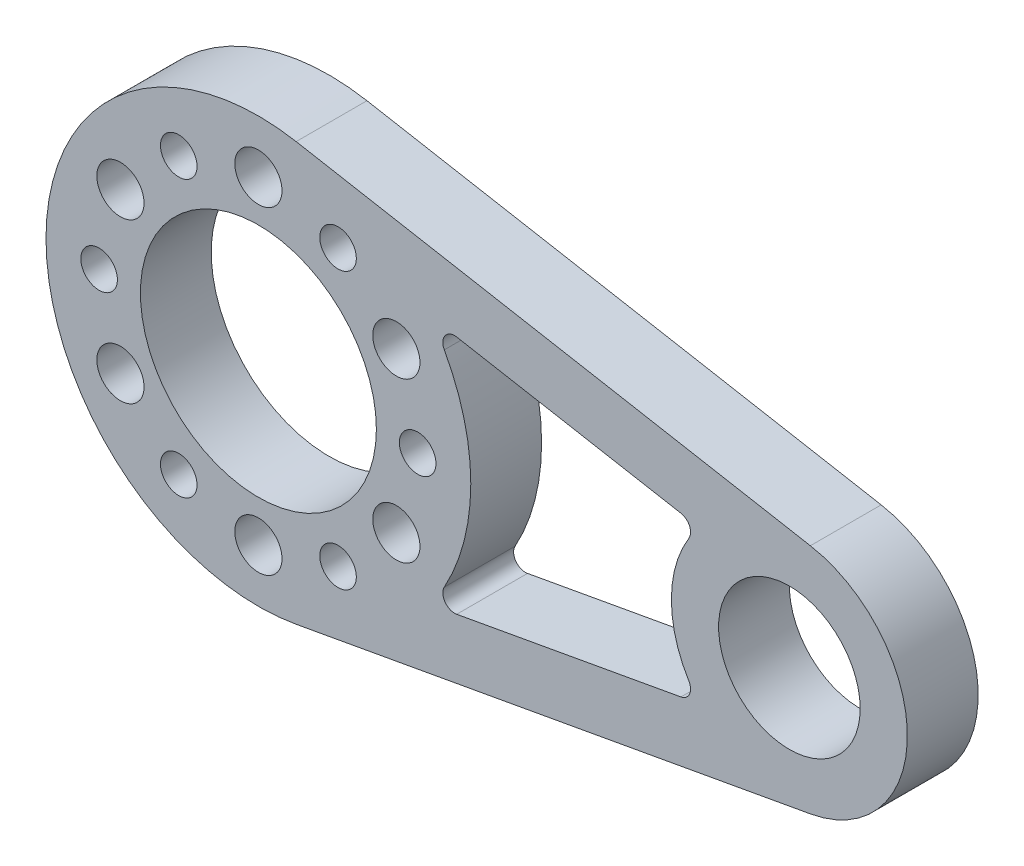
from build123d import *

# Parameters (mm, degrees)
SKETCH_1_R          = 2
SKETCH_1_R_2        = 1.55
SKETCH_1_R_3        = 10
SKETCH_1_R_4        = 6
EXTRUDE_1_DEPTH     = 6
CUT_EXTRUDE_1_DEPTH = 59.180752831
FILLET_1_R          = 1


with BuildPart() as part:
    # 草图1 → 凸台-拉伸1 (new body)
    with BuildSketch(Plane.XY):
        with BuildLine():
            Line((46.777777778, 9.840706589), (3.2, 17.71327186))
            ThreePointArc((3.2, 17.71327186), (-18, 0), (3.2, -17.71327186))
            Line((3.2, -17.71327186), (46.777777778, -9.840706589))
            ThreePointArc((46.777777778, -9.840706589), (55, 0), (46.777777778, 9.840706589))
        make_face()
        with Locations((0, 13.5)):
            Circle(SKETCH_1_R, mode=Mode.SUBTRACT)
        with Locations((6.75, 11.691342951)):
            Circle(SKETCH_1_R_2, mode=Mode.SUBTRACT)
        with Locations((0, -13.5)):
            Circle(SKETCH_1_R, mode=Mode.SUBTRACT)
        with Locations((-6.75, -11.691342951)):
            Circle(SKETCH_1_R_2, mode=Mode.SUBTRACT)
        with Locations((6.75, -11.691342951)):
            Circle(SKETCH_1_R_2, mode=Mode.SUBTRACT)
        with Locations((-11.691342951, -6.75)):
            Circle(SKETCH_1_R, mode=Mode.SUBTRACT)
        with Locations((11.691342951, -6.75)):
            Circle(SKETCH_1_R, mode=Mode.SUBTRACT)
        with Locations((-13.5, 0)):
            Circle(SKETCH_1_R_2, mode=Mode.SUBTRACT)
        Circle(SKETCH_1_R_3, mode=Mode.SUBTRACT)
        with Locations((-11.691342951, 6.75)):
            Circle(SKETCH_1_R, mode=Mode.SUBTRACT)
        with Locations((13.5, 0)):
            Circle(SKETCH_1_R_2, mode=Mode.SUBTRACT)
        with Locations((11.691342951, 6.75)):
            Circle(SKETCH_1_R, mode=Mode.SUBTRACT)
        with Locations((-6.75, 11.691342951)):
            Circle(SKETCH_1_R_2, mode=Mode.SUBTRACT)
        with Locations((45, 0)):
            Circle(SKETCH_1_R_4, mode=Mode.SUBTRACT)
    extrude(amount=EXTRUDE_1_DEPTH)

    # 草图3 → 切除-拉伸1 (cut, through all)
    with BuildSketch(Plane.XY.offset(6)):
        with BuildLine():
            Line((37.366586992, 6.459954012), (14.562692012, 10.579603082))
            ThreePointArc((14.562692012, 10.579603082), (17.119118789, 5.561993518), (18, 0))
            Line((18, 0), (35, 0))
            ThreePointArc((35, 0), (35.610268106, 3.439903336), (37.366586992, 6.459954012))
        make_face()
        with BuildLine():
            Line((35, 0), (18, 0))
            ThreePointArc((18, 0), (17.119118789, -5.561993518), (14.562692012, -10.579603082))
            Line((14.562692012, -10.579603082), (37.366586992, -6.459954012))
            ThreePointArc((37.366586992, -6.459954012), (35.610268106, -3.439903336), (35, 0))
        make_face()
    extrude(amount=-CUT_EXTRUDE_1_DEPTH, mode=Mode.SUBTRACT)

    # 圆角1
    fillet_1_edges = [part.edges().sort_by_distance(p)[0] for p in [
        (14.562692012, -10.579603082, 3),
        (14.562692012, 10.579603082, 3),
        (37.366586992, 6.459954012, 3),
        (37.366586992, -6.459954012, 3),
    ]]
    fillet(fillet_1_edges, radius=FILLET_1_R)


solid = part.part
